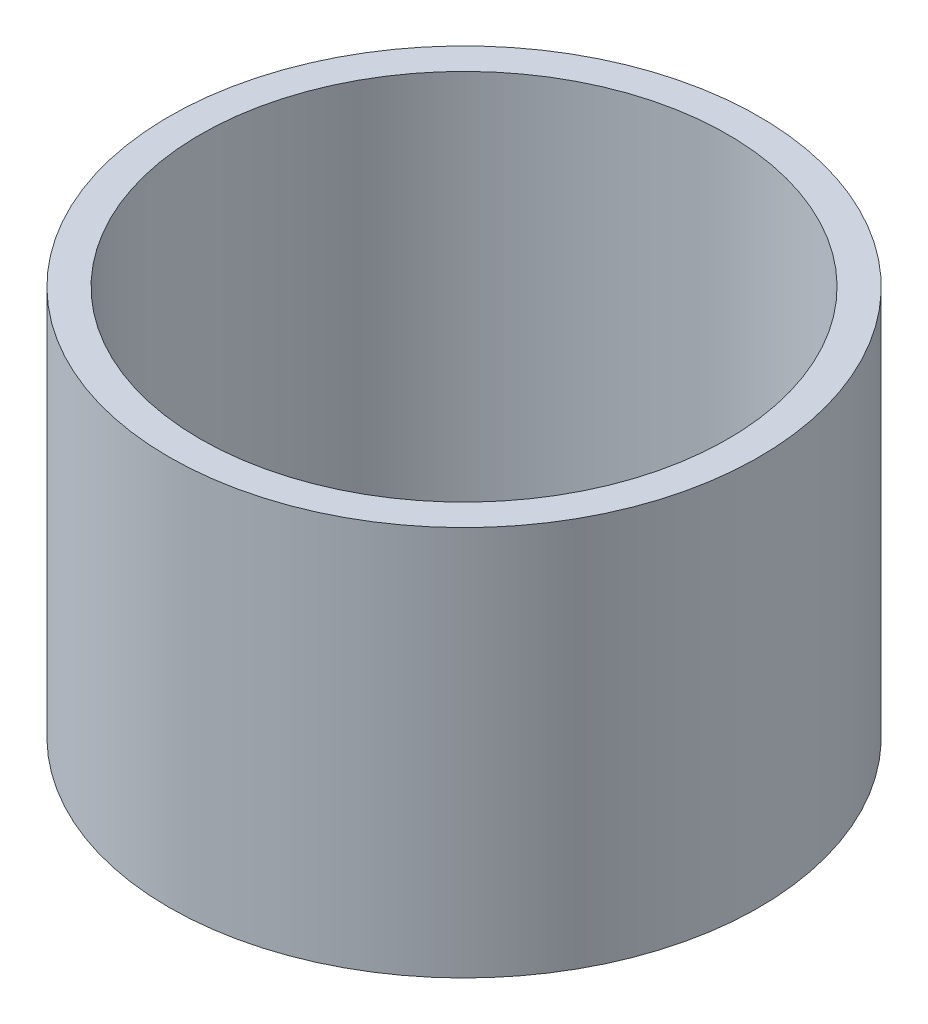
from build123d import *

# Parameters (mm, degrees)
SKETCH1_R           = 30.25
SKETCH1_R_2         = 27.05
BOSS_EXTRUDE1_DEPTH = 40


with BuildPart() as part:
    # Sketch1 → Boss-Extrude1 (new body)
    with BuildSketch(Plane(origin=(0, 0, 0), x_dir=(1, 0, 0), z_dir=(0, 1, 0))):
        with Locations(Location((0, 0, 0), (0, 0, 270))):
            Circle(SKETCH1_R)
        with Locations(Location((0, 0, 0), (0, 0, 270))):
            Circle(SKETCH1_R_2, mode=Mode.SUBTRACT)
    extrude(amount=BOSS_EXTRUDE1_DEPTH)


solid = part.part
